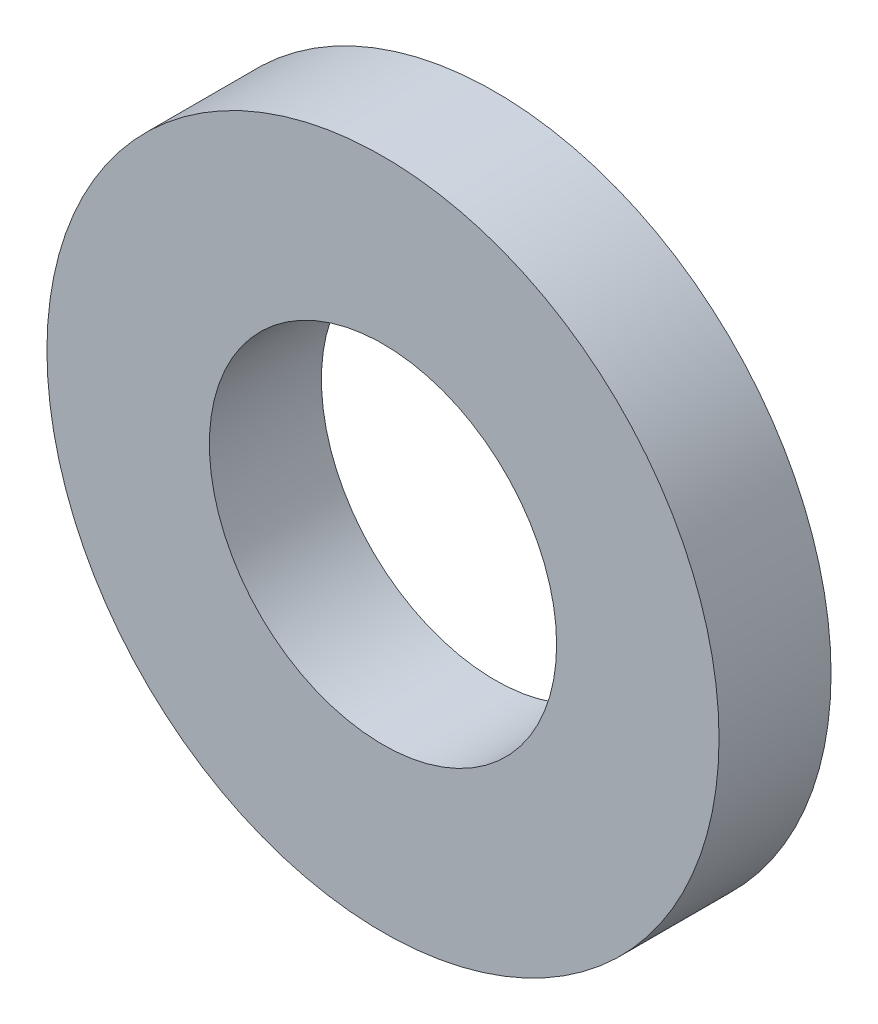
from build123d import *

# Parameters (mm, degrees)
SKETCH1_R      = 6
SKETCH1_R_2    = 3.1
EXTRUDE1_DEPTH = 2


with BuildPart() as part:
    # Sketch1 → Extrude1 (new body)
    with BuildSketch(Plane.XY):
        Circle(SKETCH1_R)
        Circle(SKETCH1_R_2, mode=Mode.SUBTRACT)
    extrude(amount=EXTRUDE1_DEPTH)


solid = part.part
